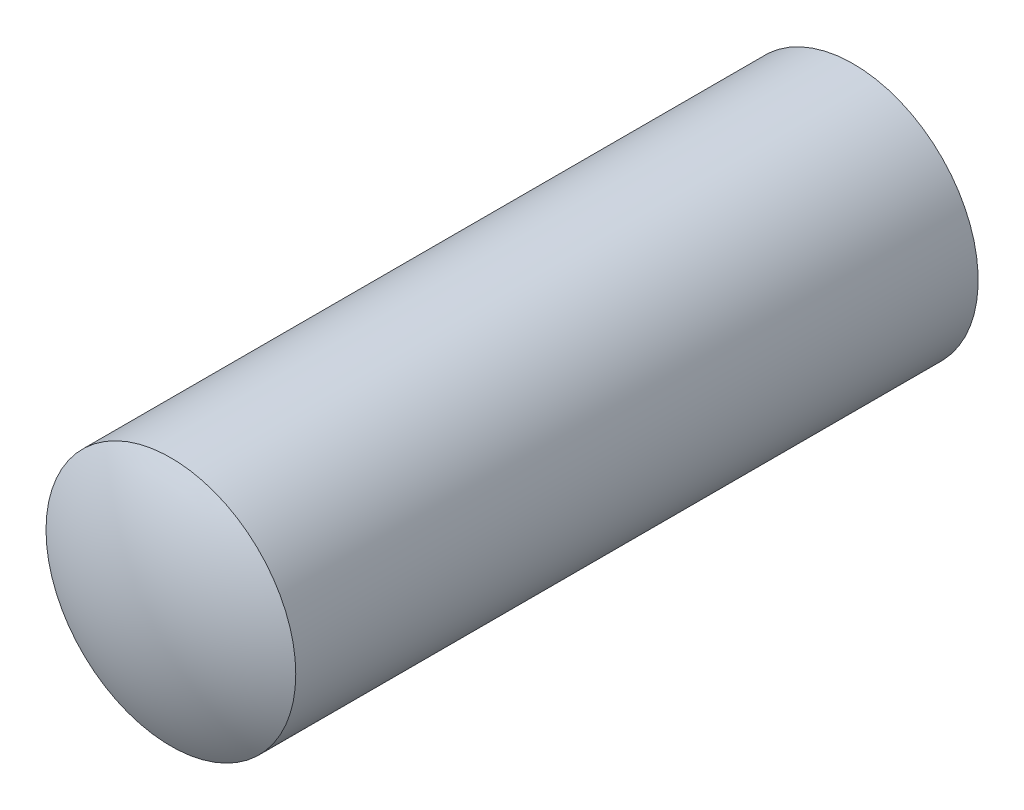
SolidWorks part; units mm, degrees
ref_plane "Front" through (0, 0, 0) normal (0, 0, 1) x (1, 0, 0)
ref_plane "Top" through (0, 0, 0) normal (0, 1, 0) x (1, 0, 0)
ref_plane "Right" through (0, 0, 0) normal (1, 0, 0) x (0, 0, -1)
sketch "Logo3_Revol_Axis" plane through (0, 0, 0) normal (0, 1, 0) x (1, 0, 0)
  line L0 (0, -30.1653) -> (0, 30.1653) construction
sketch "Logo3_bib1" plane through (0, 0, 0) normal (0, -1, 0) x (-1, 0, 0)
  line L0 (0, 8) -> (0, -4)
  line L1 (2, 7.4641) -> (2, -3.4641)
  line L10 (0, 47.5372) -> (0, -34.1764) construction
  arc A0 (2, 7.4641) -> (0, 8) centre (0, 4) ccw
  arc A1 (0, -4) -> (2, -3.4641) centre (0, 0) ccw
revolve "Revolve1" add sketch "Logo3_bib1" angle 360 about L10
equation "\"ray2@XZQB7_bib1\" = \"XZQB7_d1@XZQB7_bib1\""
equation "\"Ray1@XZQB7_bib1\" = \"XZQB7_d1@XZQB7_bib1\""
equation "\"dia1@XZQB7_bib1\" = \"XZQB7_d1@XZQB7_bib1\"/2"
